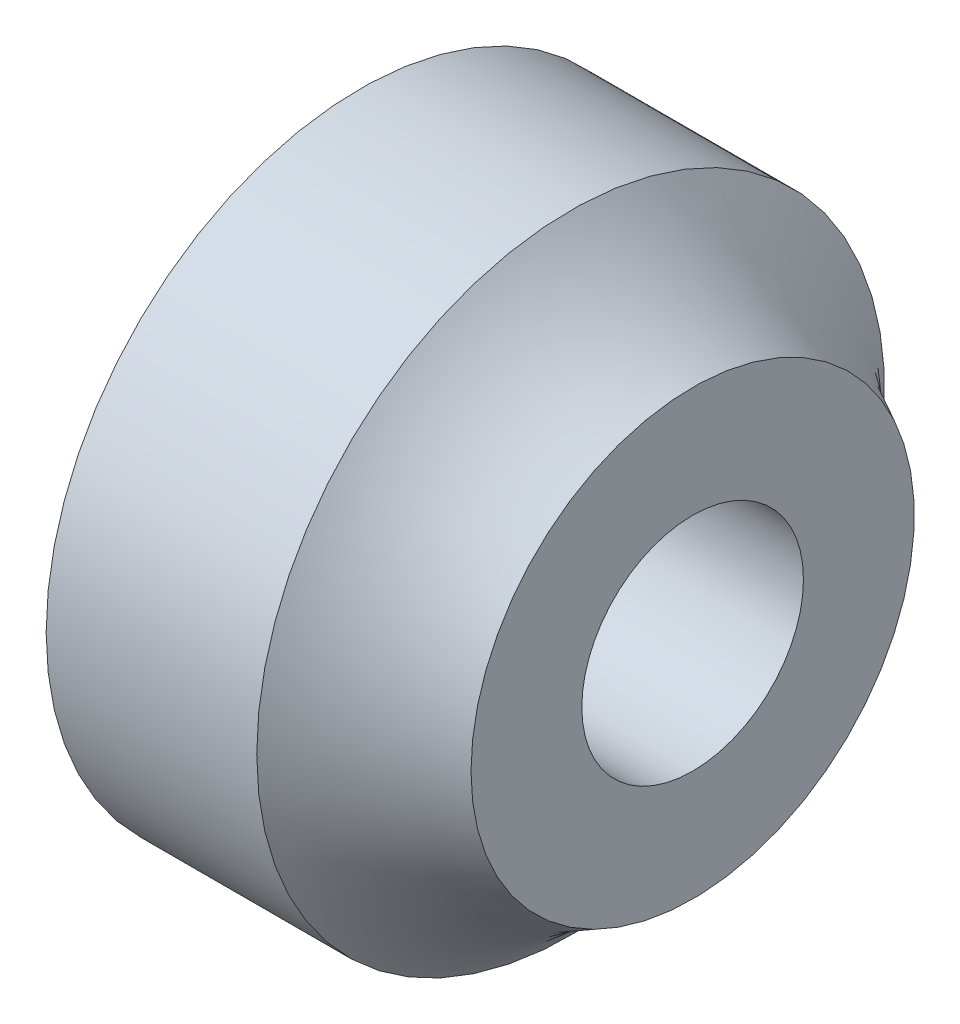
SolidWorks part; units mm, degrees
ref_plane "Front Plane" through (0, 0, 0) normal (0, 0, 1) x (1, 0, 0)
ref_plane "Top Plane" through (0, 0, 0) normal (0, 1, 0) x (1, 0, 0)
ref_plane "Right Plane" through (0, 0, 0) normal (1, 0, 0) x (0, 0, -1)
other "Configuration Table"
sketch "Sketch1" plane through (0, 0, 0) normal (0, 0, 1) x (1, 0, 0)
  line L0 (0, 0) -> (67.9568, 0) construction
  line L1 (0, 0) -> (0, 17)
  line L2 (0, 17) -> (11.4, 17)
  line L3 (18, 12) -> (18, 0)
  line L4 (18, 0) -> (0, 0)
  arc A1 (11.4, 17) -> (18, 12) centre (24.9675, 28.0531) ccw
  dimension "D1" = 34
  dimension "D2" = 11.4
  dimension "D5" = 17.5
  dimension "D4" = 24
  dimension "D3" = 18
revolve "Revolve1" add sketch "Sketch1" angle 360 about L0
sketch "Sketch2" plane through (18, 0, 0) normal (1, 0, 0) x (0, 0, -1)
  circle A0 centre (0, 0) radius 6
  dimension "D1" = 12
extrude "Cut-Extrude1" cut sketch "Sketch2" against normal through all both and the other way through all
